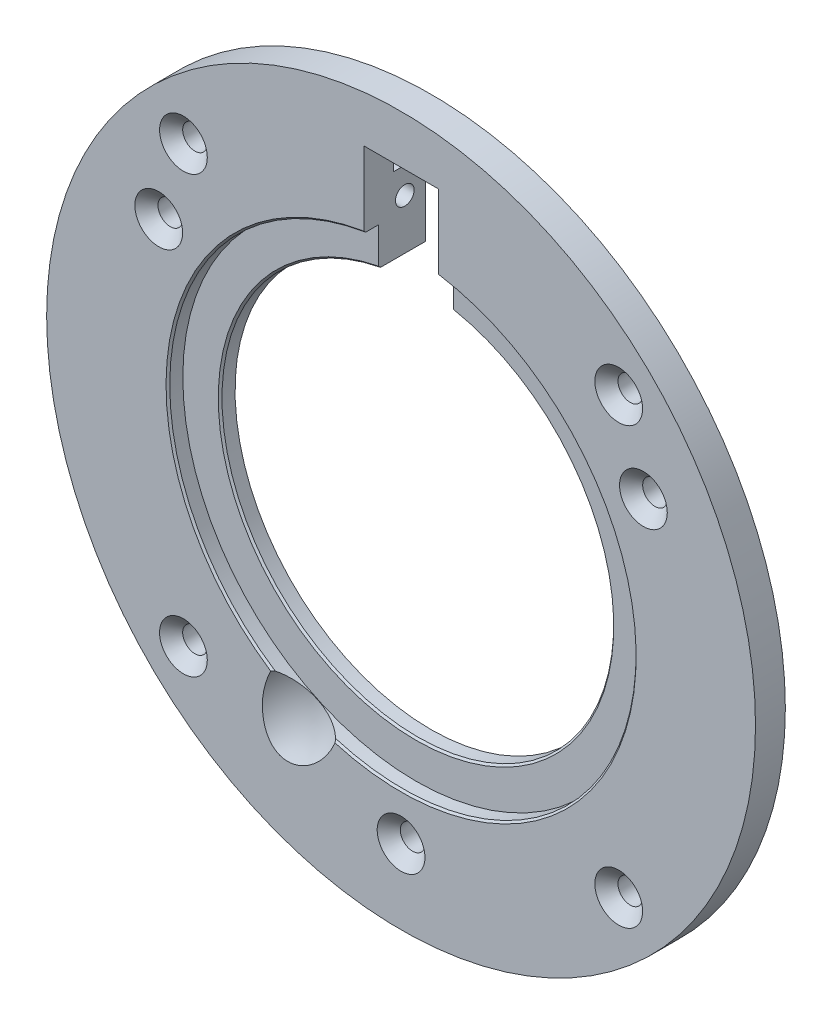
SolidWorks part; units mm, degrees
ref_plane "前视基准面" through (0, 0, 0) normal (0, 0, 1) x (1, 0, 0)
ref_plane "上视基准面" through (0, 0, 0) normal (0, 1, 0) x (1, 0, 0)
ref_plane "右视基准面" through (0, 0, 0) normal (1, 0, 0) x (0, 0, -1)
sketch "草图1" plane through (0, 0, 0) normal (0, 0, 1) x (1, 0, 0)
  circle A0 centre (0, 0) radius 95
  circle A1 centre (0, 0) radius 52.5
  dimension "D1" = 190
  dimension "D2" = 105
extrude "凸台-拉伸1" add sketch "草图1" along normal blind 8
sketch "草图3" plane through (0, 0, 8) normal (0, 0, 1) x (1, 0, 0)
  line L0 (0, 0) -> (0, 93.8899) construction
  circle A0 centre (0, 0) radius 62.5
  dimension "D1" = 125
extrude "切除-拉伸1" cut sketch "草图3" against normal blind 4
sketch "草图4" plane through (0, 0, 8) normal (0, 0, 1) x (1, 0, 0)
  line L0 (0, 0) -> (0, -82.5) construction
  line L1 (0, 0) -> (-58.3363, -58.3363) construction
  circle A0 centre (0, 0) radius 75 construction
  circle A1 centre (0, 0) radius 82.5 construction
  dimension "D1" = 150
  dimension "D2" = 165
  dimension "D3" = 45
hole_wizard "打孔尺寸(%根据)内六角花形半沉头螺钉的类型1" positions "3D草图1" profile "草图5" countersink size "M6" standard "GB"
sketch3d "3D草图1"
  line L0 (0, 0, 8) -> (0, -82.5, 8) construction
  circle A0 centre (0, 0, 8) radius 75 construction
  point P0 (0, -75, 8)
  point P6 (0, 0, 83)
sketch "草图5" plane through (0, -75, 8) normal (1, 0, 0) x (0, -1, 0)
  line L0 (0, 0) -> (0, 26.4828)
  line L1 (0, 26.4828) -> (3.3, 24.5)
  line L2 (3.3, 24.5) -> (3.3, 3.1)
  line L3 (3.3, 3.1) -> (6.4, 0)
  line L5 (6.4, 0) -> (0, 0)
  line L6 (-3.3, 3.1) -> (-6.4, 0) construction
  line L10 (0, 26.4828) -> (-3.3, 24.5) construction
  line L11 (0, -6.35) -> (0, 107.95) construction
  dimension "孔直径" = 6.6
  dimension "孔深度" = 24.5
  dimension "近端锥形沉头孔直径" = 12.8
  dimension "近端锥形沉头孔角度" = 90
  dimension "导头角度" = 118
hole_wizard "打孔尺寸(%根据)内六角花形半沉头螺钉的类型2" positions "3D草图2" profile "草图6" countersink size "M6" standard "GB"
sketch3d "3D草图2"
  point P0 (-58.3363, -58.3363, 8)
sketch "草图6" plane through (-58.3363, -58.3363, 8) normal (1, 0, 0) x (0, -1, 0)
  line L0 (0, 0) -> (0, 26.4828)
  line L1 (0, 26.4828) -> (3.3, 24.5)
  line L2 (3.3, 24.5) -> (3.3, 3.1)
  line L3 (3.3, 3.1) -> (6.4, 0)
  line L5 (6.4, 0) -> (0, 0)
  line L6 (-3.3, 3.1) -> (-6.4, 0) construction
  line L10 (0, 26.4828) -> (-3.3, 24.5) construction
  line L11 (0, -6.35) -> (0, 107.95) construction
  dimension "孔直径" = 6.6
  dimension "孔深度" = 24.5
  dimension "近端锥形沉头孔直径" = 12.8
  dimension "近端锥形沉头孔角度" = 90
  dimension "导头角度" = 118
pattern_circular "阵列(圆周)1" count 3 over 360 about axis through (0, 0, 0) along (0, 0, 1) of "打孔尺寸(%根据)内六角花形半沉头螺钉的类型1"
pattern_circular "阵列(圆周)2" count 4 over 360 about axis through (0, 0, 0) along (0, 0, 1) of "打孔尺寸(%根据)内六角花形半沉头螺钉的类型2"
sketch "草图7" plane through (0, 0, 8) normal (0, 0, 1) x (1, 0, 0)
  line L1 (-10, 82) -> (10, 82)
  line L2 (-10, 82) -> (-10, 43)
  line L3 (-10, 43) -> (10, 43)
  line L4 (10, 82) -> (10, 43)
  line L5 (-10, 82) -> (10, 43) construction
  line L6 (-10, 43) -> (10, 82) construction
  circle A0 centre (0, 0) radius 62.5 construction
  circle A1 centre (0, 0) radius 52.5 construction
  circle A2 centre (0, 0) radius 62.5 construction
  point P0 (0, 62.5)
  dimension "D1" = 20
  dimension "D2" = 82
  dimension "D3" = 10
extrude "切除-拉伸2" cut sketch "草图7" against normal blind 10
sketch "草图8" plane through (0, 0, 0) normal (0, 0, -1) x (-1, 0, 0)
  line L0 (10, 72) -> (18, 72)
  line L1 (18, 72) -> (18, 49.3178)
  line L2 (-10, 72) -> (-18, 72)
  line L3 (-18, 72) -> (-18, 49.3178)
  line L4 (-10, 51.5388) -> (-10, 82) construction
  line L5 (10, 82) -> (10, 51.5388) construction
  line L6 (-10, 72) -> (-10, 51.5388)
  line L7 (10, 72) -> (10, 51.5388)
  arc A0 (18, 49.3178) -> (10, 51.5388) centre (0, 0) ccw
  arc A1 (-10, 51.5388) -> (-18, 49.3178) centre (0, 0) ccw
  point P8 (0, 0)
  point P12 (0, 0)
  point P17 (0, 0)
  dimension "D1" = 8
  dimension "D2" = 8
  dimension "D3" = 72
extrude "凸台-拉伸2" add sketch "草图8" along normal blind 8.5
sketch "草图9" plane through (18, 0, 0) normal (1, 0, 0) x (0, 0, -1)
  line L0 (0, -95) -> (0, 95) construction
  circle A0 centre (3, 65) radius 2.5
  dimension "D1" = 5
  dimension "D2" = 3
  dimension "D3" = 65
extrude "切除-拉伸3" cut sketch "草图9" against normal through all
chamfer "倒角1" distance 0.5 angle 45 2 edges at (0, -52.5, 4) (0, -62.5, 8)
sketch "草图11" plane through (0, 0, 0) normal (0, 1, 0) x (1, 0, 0)
  line L0 (0, 0) -> (0, 65.6274) construction
ref_plane "基准面1" through (0, 0, 0) normal (-0.9063, 0.4226, 0) x (0, 0, -1)
sketch "草图12" plane through (0, 0, 0) normal (-0.9063, 0.4226, 0) x (0, 0, -1)
  line L0 (-17.5, 88) -> (-17.5, 38)
  line L1 (-4, 31.0701) -> (-4, 118.0787) construction
  line L2 (-8, 95) -> (-8, -95) construction
  line L3 (0, 0) -> (-56.2666, 0) construction
  line L4 (-4, 63) -> (-23.3904, 63) construction
  line L6 (-17.5, 88) -> (-17.5, 38) construction
  arc A0 (-17.5, 88) -> (-17.5, 38) centre (-34.0193, 63) cw
  dimension "D1" = 4
  dimension "D2" = 63
  dimension "D4" = 13.5
  dimension "D5" = 50
  dimension "D6" = 25
revolve "切除-旋转1" cut sketch "草图12" angle 360 about L6
